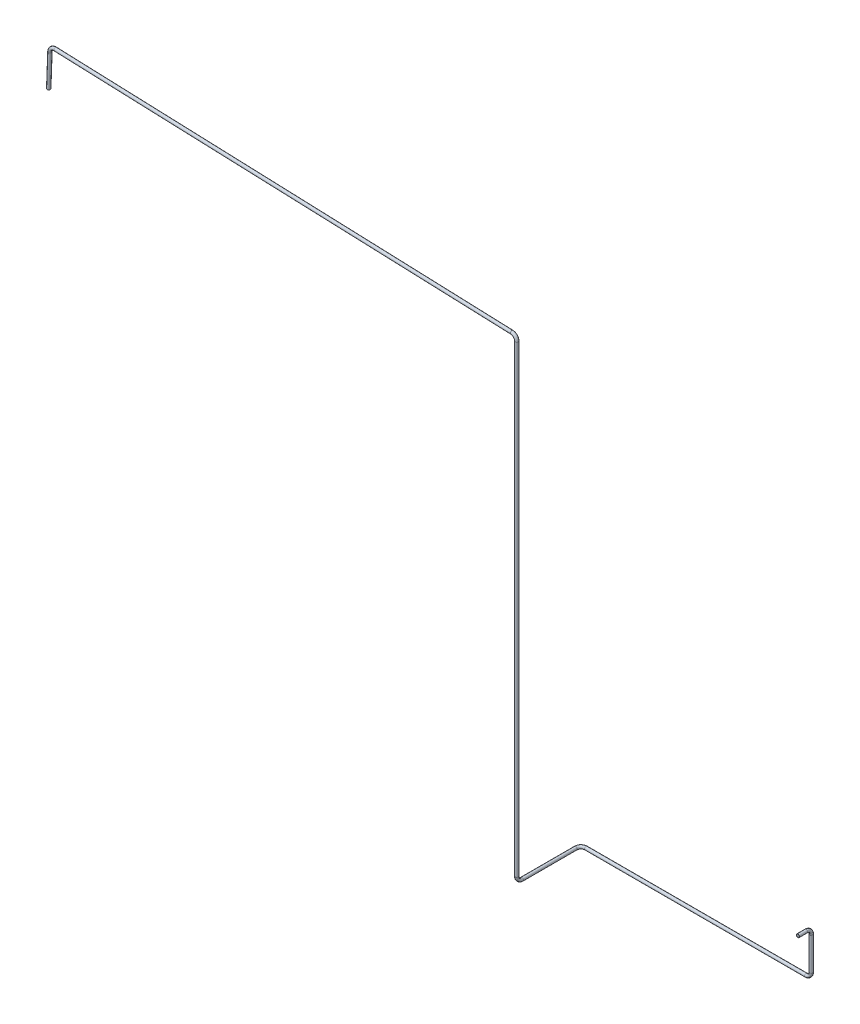
from build123d import *

# Parameters (mm, degrees)
SWEEP_1_PROFILE_R   = 6
SWEEP_1_PROFILE_R_2 = 5


with BuildPart() as part:
    # 扫描-薄件1: sweep along a curve in space
    with BuildLine() as sweep_1_path:
        Line((1880.512693362, 1290.797471808, 260.319452586), (1880.512693362, 1290.797471808, 229.002272719))
        ThreePointArc((1880.512693362, 1270.797471808, 209.002272719), (1880.512693362, 1284.939607432, 214.860137095), (1880.512693362, 1290.797471808, 229.002272719))
        Line((1880.512693362, 1270.797471808, 209.002272719), (1880.512693362, 1144.670229131, 209.002272719))
        ThreePointArc((1860.512693362, 1124.670229131, 209.002272719), (1874.654828986, 1130.528093508, 209.002272719), (1880.512693362, 1144.670229131, 209.002272719))
        Line((1860.512693362, 1124.670229131, 209.002272719), (1017.606912513, 1124.670229131, 209.002272719))
        ThreePointArc((997.606912513, 1124.670229131, 229.002272719), (1003.464776889, 1124.670229131, 214.860137095), (1017.606912513, 1124.670229131, 209.002272719))
        Line((997.606912513, 1124.670229131, 229.002272719), (997.606912513, 1124.670229131, 434.912562332))
        ThreePointArc((997.606912513, 1124.670229131, 434.912562332), (997.606912513, 1130.528093508, 449.054697956), (997.606912513, 1144.670229131, 454.912562332))
        Line((997.606912513, 1144.670229131, 454.912562332), (997.606912513, 2920.615742332, 454.912562332))
        ThreePointArc((997.606912513, 2920.615742332, 454.912562332), (992.009233976, 2934.492814663, 454.912562332), (978.349598866, 2940.601948, 454.912562332))
        Line((978.349598866, 2940.601948, 454.912562332), (-770.803765777, 3005.600395166, 454.912562332))
        ThreePointArc((-791.532657797, 2986.356875851, 454.912562332), (-785.153675131, 3000.271729612, 454.912562332), (-770.803765777, 3005.600395166, 454.912562332))
        Line((-791.532657797, 2986.356875851, 454.912562332), (-796.169484167, 2861.576657254, 454.912562332))
    # 扫描-薄件1 profile (on start of the path) → 扫描-薄件1 (sweep)
    with BuildSketch(Plane(origin=(1880.512693362, 1290.797471808, 260.319452586), x_dir=(-1, 0, 0), z_dir=(0, 0, -1))):
        Circle(SWEEP_1_PROFILE_R)
        Circle(SWEEP_1_PROFILE_R_2, mode=Mode.SUBTRACT)
    sweep(path=sweep_1_path.line)


solid = part.part
